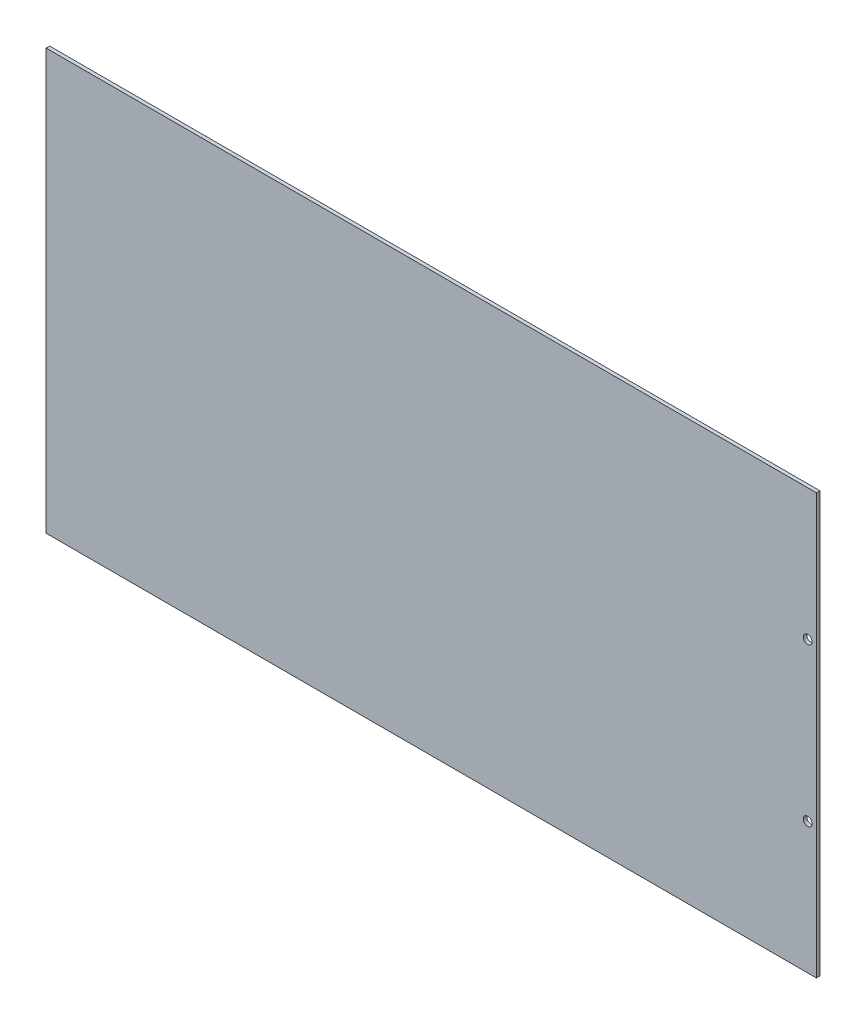
from build123d import *

# Parameters (mm, degrees)
SKETCH_1_W          = 440
SKETCH_1_H          = 240
EXTRUDE_1_DEPTH     = 2
SKETCH_2_R          = 2.5
CUT_EXTRUDE_1_DEPTH = 2


with BuildPart() as part:
    # 草图1 → 凸台-拉伸1 (new body)
    with BuildSketch(Plane.XY):
        Rectangle(SKETCH_1_W, SKETCH_1_H)
    extrude(amount=EXTRUDE_1_DEPTH)

    # 草图2 → 切除-拉伸1 (cut)
    with BuildSketch(Plane.XY.offset(2)):
        with Locations((215, 44.9966)):
            Circle(SKETCH_2_R)
        with Locations((215, -45.0034)):
            Circle(SKETCH_2_R)
    extrude(amount=-CUT_EXTRUDE_1_DEPTH, mode=Mode.SUBTRACT)


solid = part.part
